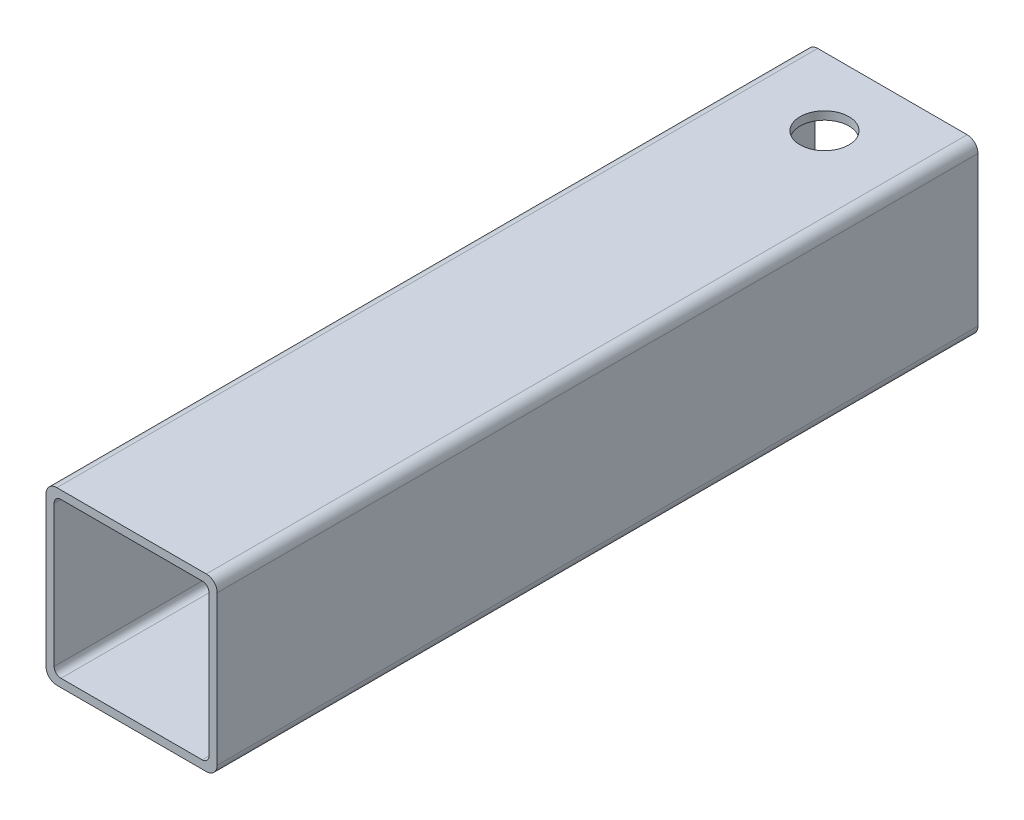
from build123d import *

# Parameters (mm, degrees)
SKETCH1_W           = 126
SKETCH1_H           = 126
SKETCH1_W_2         = 114
SKETCH1_H_2         = 114
BOSS_EXTRUDE1_DEPTH = 560
FILLET1_R           = 8
FILLET2_R           = 5
SKETCH3_R           = 18
CUT_EXTRUDE1_DEPTH  = 260


with BuildPart() as part:
    # Sketch1 → Boss-Extrude1 (new body)
    with BuildSketch(Plane.XY):
        with Locations((63, 63)):
            Rectangle(SKETCH1_W, SKETCH1_H)
        with Locations((63, 63)):
            Rectangle(SKETCH1_W_2, SKETCH1_H_2, mode=Mode.SUBTRACT)
    extrude(amount=BOSS_EXTRUDE1_DEPTH)

    # Fillet1
    fillet1_edges = [part.edges().sort_by_distance(p)[0] for p in [
        (0, 126, 280),
        (126, 126, 280),
        (126, 0, 280),
        (0, 0, 280),
    ]]
    fillet(fillet1_edges, radius=FILLET1_R)

    # Fillet2
    fillet2_edges = [part.edges().sort_by_distance(p)[0] for p in [
        (6, 120, 280),
        (6, 6, 280),
        (120, 6, 280),
        (120, 120, 280),
    ]]
    fillet(fillet2_edges, radius=FILLET2_R)

    # Sketch3 → Cut-Extrude1 (cut)
    with BuildSketch(Plane.XZ):
        with Locations(Location((63, 50, 0), (0, 0, 270))):
            Circle(SKETCH3_R)
    extrude(amount=-CUT_EXTRUDE1_DEPTH, mode=Mode.SUBTRACT)


solid = part.part
